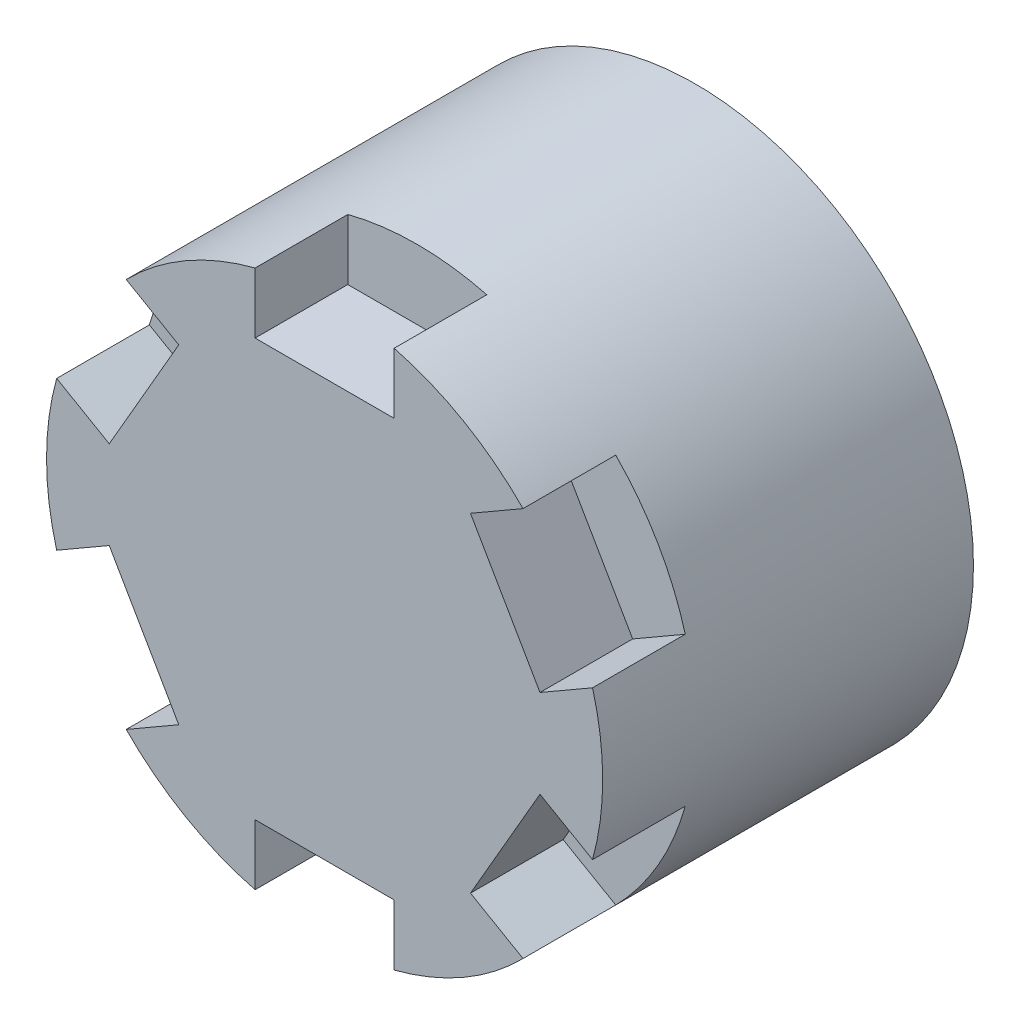
SolidWorks part; units mm, degrees
ref_plane "前视基准面" through (0, 0, 0) normal (0, 0, 1) x (1, 0, 0)
ref_plane "上视基准面" through (0, 0, 0) normal (0, 1, 0) x (1, 0, 0)
ref_plane "右视基准面" through (0, 0, 0) normal (1, 0, 0) x (0, 0, -1)
other "Configuration Table"
sketch "草图1" plane through (0, 0, 0) normal (0, 0, 1) x (1, 0, 0)
  circle A0 centre (0, 0) radius 37.5
  dimension "D1" = 75
sketch "草图2" plane through (0, 0, 0) normal (0, 0, 1) x (1, 0, 0)
  circle A0 centre (0, 0) radius 60
  dimension "D1" = 120
extrude "凸台-拉伸1" add sketch "草图2" along normal blind 80 contours A0
extrude "切除-拉伸1" cut sketch "草图1" along normal blind 60 contours A0
sketch "草图3" plane through (0, 0, 80) normal (0, 0, 1) x (1, 0, 0)
  line L0 (57.8115, 16.057) -> (46.4711, 9.5096)
  line L2 (-15, 58.0948) -> (-15, 45)
  line L3 (-15, 45) -> (15, 45)
  line L4 (15, 58.0948) -> (15, 45)
  line L5 (31.4711, 35.4904) -> (46.4711, 9.5096)
  line L6 (42.8115, 42.0378) -> (31.4711, 35.4904)
  line L7 (42.8115, -42.0378) -> (31.4711, -35.4904)
  line L8 (46.4711, -9.5096) -> (31.4711, -35.4904)
  line L9 (57.8115, -16.057) -> (46.4711, -9.5096)
  line L10 (-15, -58.0948) -> (-15, -45)
  line L11 (15, -45) -> (-15, -45)
  line L12 (15, -58.0948) -> (15, -45)
  line L13 (-57.8115, -16.057) -> (-46.4711, -9.5096)
  line L14 (-31.4711, -35.4904) -> (-46.4711, -9.5096)
  line L15 (-42.8115, -42.0378) -> (-31.4711, -35.4904)
  line L16 (-42.8115, 42.0378) -> (-31.4711, 35.4904)
  line L17 (-46.4711, 9.5096) -> (-31.4711, 35.4904)
  line L18 (-57.8115, 16.057) -> (-46.4711, 9.5096)
  circle A0 centre (0, 0) radius 60 construction
  arc A1 (15, 58.0948) -> (-15, 58.0948) centre (0, 0) ccw
  arc A2 (57.8115, 16.057) -> (42.8115, 42.0378) centre (0, 0) ccw
  arc A3 (42.8115, -42.0378) -> (57.8115, -16.057) centre (0, 0) ccw
  arc A4 (-15, -58.0948) -> (15, -58.0948) centre (0, 0) ccw
  arc A5 (-57.8115, -16.057) -> (-42.8115, -42.0378) centre (0, 0) ccw
  arc A6 (-42.8115, 42.0378) -> (-57.8115, 16.057) centre (0, 0) ccw
  point P7 (0, 45)
  dimension "D1" = 30
  dimension "D2" = 45
  dimension "D3" = 6
extrude "切除-拉伸2" cut sketch "草图3" against normal blind 20
sketch "草图4" plane through (0, 0, 0) normal (0, 0, -1) x (-1, 0, 0)
  line L1 (-10, 40) -> (10, 40)
  line L2 (-10, 40) -> (-10, 28.3316)
  line L3 (-10, 28.3316) -> (10, 28.3316)
  line L4 (10, 40) -> (10, 28.3316)
  point P4 (0, 28.3316)
  dimension "D1" = 20
  dimension "D2" = 40
extrude "切除-拉伸3" cut sketch "草图4" against normal blind 30 contours L4 L3 L2 L1
